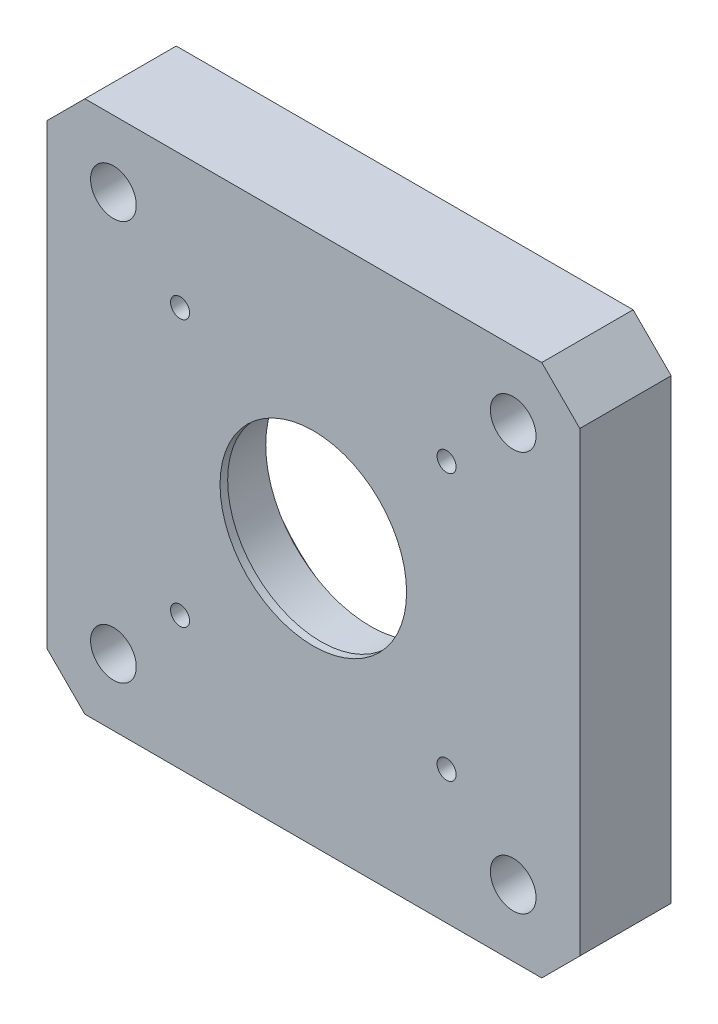
SolidWorks part; units mm, degrees
material "6061Al"
ref_plane "前视基准面" through (0, 0, 0) normal (0, 0, 1) x (1, 0, 0)
ref_plane "上视基准面" through (0, 0, 0) normal (0, 1, 0) x (1, 0, 0)
ref_plane "右视基准面" through (0, 0, 0) normal (1, 0, 0) x (0, 0, -1)
sketch "草图1" plane through (0, 0, 0) normal (0, 0, 1) x (1, 0, 0)
  line L1 (-70, -70) -> (70, -70)
  line L2 (-70, -70) -> (-70, 70)
  line L3 (-70, 70) -> (70, 70)
  line L4 (70, -70) -> (70, 70)
  line L5 (-70, -70) -> (70, 70) construction
  line L6 (-70, 70) -> (70, -70) construction
  point P0 (0, 0)
  dimension "D1" = 140
extrude "凸台-拉伸1" add sketch "草图1" along normal blind 24
sketch "草图2" plane through (0, 0, 0) normal (0, 0, -1) x (-1, 0, 0)
  circle A0 centre (0, 0) radius 27.5
  dimension "D1" = 55
extrude "切除-拉伸1" cut sketch "草图2" against normal offset from surface (22 mm away) 2 up to face at (0, 0, 24)
sketch "草图3" plane through (0, 0, 22) normal (0, 0, -1) x (-1, 0, 0)
  circle A0 centre (0, 0) radius 24.5
  circle A2 centre (0, 0) radius 27.5 construction
  dimension "D1" = 3
extrude "切除-拉伸2" cut sketch "草图3" against normal through all
hole_wizard "M10 六角凹头螺钉的柱形沉头孔1" positions "草图7" profile "草图8" counterbore size "M10" standard "ISO" end condition through all
sketch "草图7" plane through (0, 0, 0) normal (0, 0, -1) x (-1, 0, 0)
  line L0 (0, 0) -> (0, 70) construction
  line L1 (-70, 70) -> (70, 70) construction
  line L3 (0, 0) -> (70, 0) construction
  line L4 (70, 70) -> (70, -70) construction
  point P0 (-52.5, 52.5)
  point P17 (52.5, 52.5)
  point P18 (52.5, -52.5)
  point P19 (-52.5, -52.5)
  dimension "D1" = 105
  dimension "D2" = 105
sketch "草图8" plane through (52.5, 52.5, 0) normal (1, 0, 0) x (0, 1, 0)
  line L0 (0, 0) -> (0, 24)
  line L1 (0, 24) -> (6, 24)
  line L3 (6, 24) -> (6, 10.6)
  line L4 (6, 10.6) -> (9, 10.6)
  line L5 (9, 10.6) -> (9, 0)
  line L7 (9, 0) -> (0, 0)
  line L11 (0, -6.35) -> (0, 107.95) construction
  dimension "通孔孔直径" = 12
  dimension "通孔孔深度" = 24
  dimension "柱形沉头孔直径" = 18
  dimension "柱形沉头孔深度" = 10.6
chamfer "倒角1" distance 10 angle 45 4 edges at (70, -70, 12) (-70, -70, 12) (-70, 70, 12) (70, 70, 12)
hole_wizard "M6 螺纹孔1" positions "草图9" profile "草图10" tap size "M6" standard "ISO" end condition through all
sketch "草图9" plane through (0, 0, 0) normal (0, 0, -1) x (-1, 0, 0)
  line L1 (-35, -35) -> (35, -35)
  line L2 (-35, -35) -> (-35, 35)
  line L3 (-35, 35) -> (35, 35)
  line L4 (35, -35) -> (35, 35)
  line L5 (-35, -35) -> (35, 35) construction
  line L6 (-35, 35) -> (35, -35) construction
  point P0 (-35, 35)
  point P3 (35, 35)
  point P6 (35, -35)
  point P9 (-35, -35)
  point P13 (0, 0)
  dimension "D1" = 70
sketch "草图10" plane through (35, 35, 0) normal (1, 0, 0) x (0, 1, 0)
  line L0 (0, 0) -> (0, 24)
  line L1 (0, 24) -> (2.5, 24)
  line L2 (2.5, 24) -> (2.5, 0)
  line L5 (2.5, 0) -> (0, 0)
  line L11 (0, -6.35) -> (0, 107.95) construction
  dimension "通孔螺纹孔钻头直径" = 5
  dimension "通孔螺纹孔钻头深度" = 24
cosmetic thread "孔螺蚊线1" parameters "D2"=6
cosmetic thread "孔螺蚊线2" parameters "D2"=6
cosmetic thread "孔螺蚊线3" parameters "D2"=6
cosmetic thread "孔螺蚊线4" parameters "D2"=6
sketch "草图11" plane through (0, 0, 0) normal (0, 0, -1) x (-1, 0, 0)
  circle A0 centre (0, 0) radius 40
  dimension "D1" = 80
extrude "切除-拉伸3" cut sketch "草图11" against normal blind 9
sketch "草图16" plane through (0, 0, 9) normal (0, 0, -1) x (-1, 0, 0)
  line L0 (0, 30.5) -> (0, 0) construction
  line L1 (0, 0) -> (0, 30.5) construction
  circle A0 centre (0, 30.5) radius 6
  circle A4 centre (0, 0) radius 27.5 construction
  circle A5 centre (30.5, 0) radius 6
  circle A6 centre (0, -30.5) radius 6
  circle A7 centre (-30.5, 0) radius 6
  dimension "D1" = 12
  dimension "D2" = 3
  dimension "D3" = 4
extrude "切除-拉伸4" [suppressed] cut sketch "草图16" against normal blind 3.5
hole_wizard "M5 螺纹孔1" positions "草图17" profile "草图18" tap size "M5" standard "ISO"
sketch "草图17" [suppressed] plane through (0, 0, 11) normal (0, 0, -1) x (-1, 0, 0)
  point P0 (0, 26.5)
  point P3 (25.6098, 0)
  point P5 (0, -26.5)
  point P8 (-26.5, 0)
sketch "草图18" plane through (0, 26.5, 11) normal (1, 0, 0) x (0, 1, 0)
  line L0 (0, 0) -> (0, 11)
  line L1 (0, 11) -> (2.1, 11)
  line L2 (2.1, 11) -> (2.1, 0)
  line L5 (2.1, 0) -> (0, 0)
  line L11 (0, -6.35) -> (0, 107.95) construction
  dimension "通孔螺纹孔钻头直径" = 4.2
  dimension "通孔螺纹孔钻头深度" = 11
cosmetic thread "孔螺蚊线5" [suppressed] parameters "D2"=5
cosmetic thread "孔螺蚊线6" [suppressed] parameters "D2"=5
cosmetic thread "孔螺蚊线7" [suppressed] parameters "D2"=5
cosmetic thread "孔螺蚊线8" [suppressed] parameters "D2"=5
